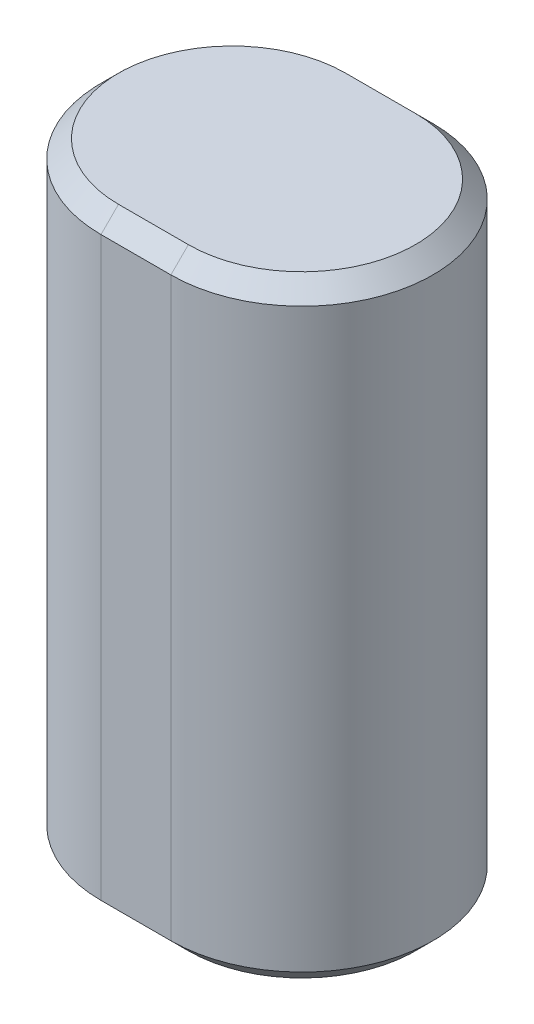
SolidWorks part; units mm, degrees
material "20#"
ref_plane "Front" through (0, 0, 0) normal (0, 0, 1) x (1, 0, 0)
ref_plane "Top" through (0, 0, 0) normal (0, 1, 0) x (1, 0, 0)
ref_plane "Right" through (0, 0, 0) normal (1, 0, 0) x (0, 0, -1)
sketch "Sketch1" plane through (0, 0, 0) normal (0, 1, 0) x (1, 0, 0)
  line L0 (-2, 0) -> (2, 0) construction
  line L1 (-2, 7.5) -> (2, 7.5)
  line L2 (-2, -7.5) -> (2, -7.5)
  arc A0 (-2, 7.5) -> (-2, -7.5) centre (-2, 0) ccw
  arc A1 (2, -7.5) -> (2, 7.5) centre (2, 0) ccw
  point P3 (0, 0)
  dimension "D1" = 7.5
  dimension "D2" = 4
extrude "Boss-Extrude1" add sketch "Sketch1" along normal blind 35
chamfer "Chamfer1" distance 1 angle 45 8 edges at (9.5, 0, 0) (0, 0, -7.5) (0, 0, 7.5) (-9.5, 0, 0) (9.5, 35, 0) (0, 35, -7.5) (0, 35, 7.5) (-9.5, 35, 0)
